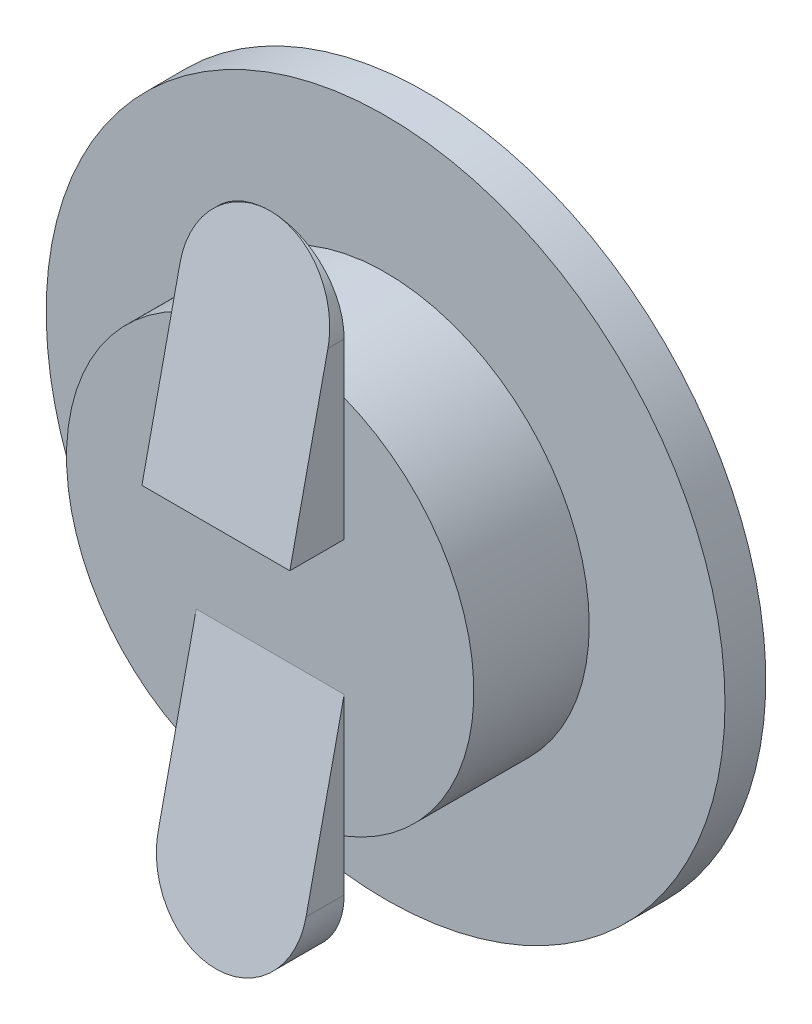
SolidWorks part; units mm, degrees
ref_plane "Front Plane" through (0, 0, 0) normal (0, 0, 1) x (1, 0, 0)
ref_plane "Top Plane" through (0, 0, 0) normal (0, 1, 0) x (1, 0, 0)
ref_plane "Right Plane" through (0, 0, 0) normal (1, 0, 0) x (0, 0, -1)
other "Configuration Table"
sketch "Sketch1" plane through (0, 0, 0) normal (0, 0, 1) x (1, 0, 0)
  circle A0 centre (0, 0) radius 25
  dimension "D1" = 50
extrude "Boss-Extrude1" add sketch "Sketch1" along normal mid plane 3
sketch "Sketch2" plane through (0, 0, -1.5) normal (0, 0, -1) x (-1, 0, 0)
  line L1 (-24.8408, 2.8167) -> (24.8408, 2.8167)
  line L2 (-90.0288, 2.8167) -> (-90.0288, -2.8167)
  line L3 (-24.8408, -2.8167) -> (24.8408, -2.8167)
  line L5 (-28.3126, -2.8167) -> (-28.3126, 2.8167) construction
  line L6 (-25, 0) -> (25, 0) construction
  circle A0 centre (0, 0) radius 25 construction
  arc A1 (-24.8408, 2.8167) -> (-24.8408, -2.8167) centre (0, 0) ccw
  arc A2 (24.8408, -2.8167) -> (24.8408, 2.8167) centre (0, 0) ccw
  point P0 (-28.3126, 0)
  circle M9 centre (0, 0) radius 25
extrude "Boss-Extrude2" add sketch "Sketch2" along normal blind 8 contours L3 L1 M9
sketch "Sketch3" plane through (0, 2.8167, 0) normal (0, 1, 0) x (1, 0, 0)
  line L0 (24.8408, 1.5) -> (29.901, 1.5)
  line L1 (29.901, 1.5) -> (29.901, 11.2999)
  line L2 (29.901, 11.2999) -> (-29.6605, 11.2999)
  line L3 (-29.6605, 11.2999) -> (-29.6605, 1.5)
  line L4 (-24.8408, 1.5) -> (24.8408, 1.5)
  line L5 (24.8408, 1.5) -> (24.8408, 9.5)
  line L6 (24.8408, 9.5) -> (-24.8408, 9.5)
  line L7 (-24.8408, 9.5) -> (-24.8408, 1.5)
  line L8 (-24.8408, 1.5) -> (24.8408, 1.5)
  line L12 (-29.6605, 1.5) -> (-24.8408, 1.5)
  arc A0 (-24.8408, 1.5) -> (24.8408, 1.5) centre (0, -36.1621) cw
  line M7 (24.8408, 1.5) -> (24.8408, 9.5)
  line M8 (24.8408, 9.5) -> (-24.8408, 9.5)
  line M9 (-24.8408, 9.5) -> (-24.8408, 1.5)
  dimension "D1" = 0
extrude "Cut-Extrude2" cut sketch "Sketch3" against normal blind 8 contours L3 L12 L0 L1 L2 M9 M8 M7 | A0 M9 M7 M8
sketch "Sketch4" plane through (0, 0, 1.5) normal (0, 0, 1) x (1, 0, 0)
  circle A0 centre (0, 0) radius 15
  dimension "D1" = 30
extrude "Boss-Extrude3" add sketch "Sketch4" along normal blind 8.5
sketch "Sketch5" plane through (0, 0, 10) normal (0, 0, 1) x (1, 0, 0)
  line L0 (0, 0) -> (45.3189, 0) construction
  line L2 (-5.4476, 17.7308) -> (-5.4476, 4.944)
  line L3 (-5.4476, 4.944) -> (5.4476, 4.944)
  line L4 (5.4476, 17.7308) -> (5.4476, 4.944)
  line L5 (0, 4.944) -> (0, 14.9995) construction
  line L6 (-5.4476, -17.7308) -> (-5.4476, -4.944)
  line L7 (-5.4476, -4.944) -> (5.4476, -4.944)
  line L8 (5.4476, -17.7308) -> (5.4476, -4.944)
  arc A2 (-5.4476, 17.7308) -> (5.4476, 17.7308) centre (0, 17.7308) cw
  arc A3 (-5.4476, -17.7308) -> (5.4476, -17.7308) centre (0, -17.7308) ccw
  point P0 (0, 19.049)
extrude "Boss-Extrude4" add sketch "Sketch5" along normal blind 4
sketch "Sketch7" plane through (-5.4476, 0, 0) normal (-1, 0, 0) x (0, 0, 1)
  line L0 (10, 23.1785) -> (14, 4.944)
  line L1 (14, -23.1785) -> (10, -4.944)
  line L2 (10, 23.1785) -> (14, 23.1785)
  line L3 (14, 17.7308) -> (14, 23.1785) construction
  line L4 (14, 23.1785) -> (14, 4.944)
  line L5 (10, -4.944) -> (14, -4.944)
  line L6 (14, -4.944) -> (14, -23.1785)
extrude "Cut-Extrude3" cut sketch "Sketch7" against normal through all
